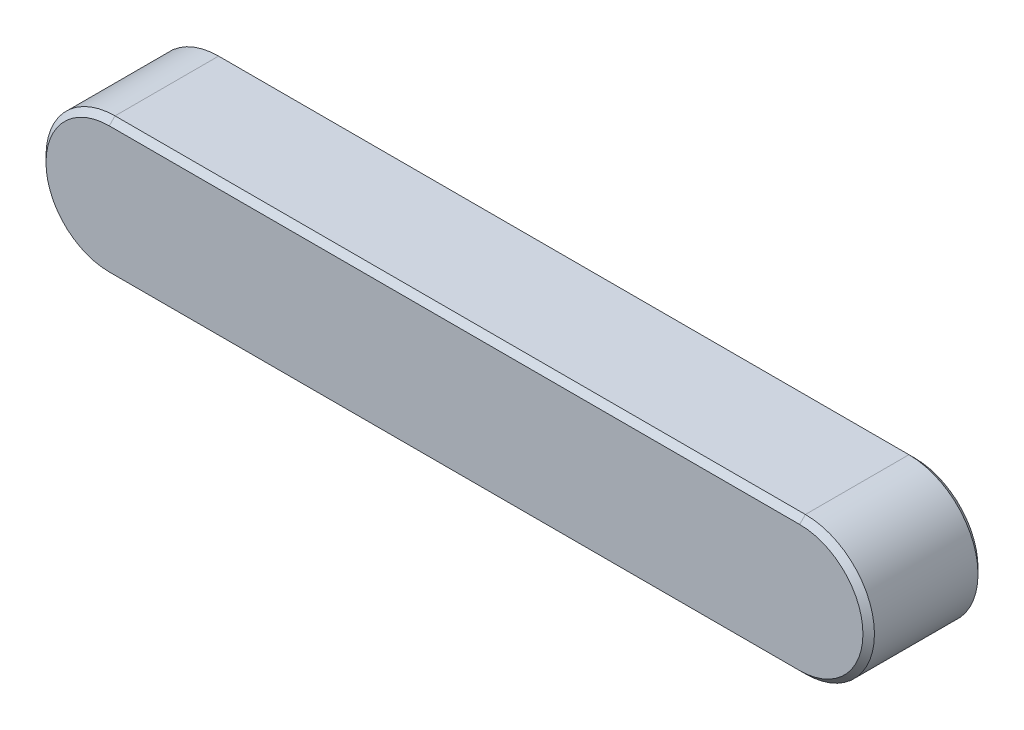
SolidWorks part; units mm, degrees
ref_plane "Front Plane" through (0, 0, 0) normal (0, 0, 1) x (1, 0, 0)
ref_plane "Top Plane" through (0, 0, 0) normal (0, 1, 0) x (1, 0, 0)
ref_plane "Right Plane" through (0, 0, 0) normal (1, 0, 0) x (0, 0, -1)
sketch "Sketch1" plane through (0, 0, 0) normal (0, 0, 1) x (1, 0, 0)
  line L0 (0, 0) -> (60, 0) construction
  line L1 (0, 6) -> (60, 6)
  line L2 (0, -6) -> (60, -6)
  arc A0 (0, 6) -> (0, -6) centre (0, 0) ccw
  arc A1 (60, -6) -> (60, 6) centre (60, 0) ccw
  point P3 (30, 0)
  dimension "D1" = 60
  dimension "D2" = 12
extrude "Boss-Extrude1" add sketch "Sketch1" along normal blind 10
chamfer "Chamfer1" distance 0.5 angle 45 8 edges at (30, -6, 0) (66, 0, 0) (30, 6, 0) (-6, 0, 0) (30, 6, 10) (66, 0, 10) (30, -6, 10) (-6, 0, 10)
